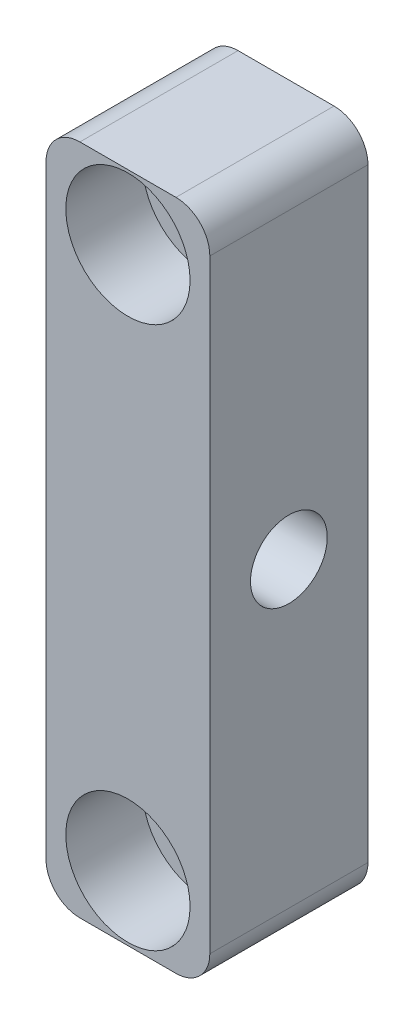
from build123d import *

# Parameters (mm, degrees)
SKETCH_1_W                = 14.5
SKETCH_1_H                = 59.5
EXTRUDE_1_DEPTH           = 14
FILLET_1_R                = 3
HOLE_WIZARD_2_D           = 6.6
HOLE_WIZARD_2_CBORE_D     = 11
HOLE_WIZARD_2_CBORE_DEPTH = 6.8
HOLE_WIZARD_M8_1_D        = 6.8


with BuildPart() as part:
    # 草图1 → 凸台-拉伸1 (new body)
    with BuildSketch(Plane.XY):
        Rectangle(SKETCH_1_W, SKETCH_1_H)
    extrude(amount=EXTRUDE_1_DEPTH)

    # 圆角1
    fillet_1_edges = [part.edges().sort_by_distance(p)[0] for p in [
        (7.25, -29.75, 7),
        (-7.25, -29.75, 7),
        (-7.25, 29.75, 7),
        (7.25, 29.75, 7),
    ]]
    fillet(fillet_1_edges, radius=FILLET_1_R)

    # 打孔尺寸(%根据)内六角圆柱头螺钉的类型2 (through all)
    with Locations(Plane.XY.offset(14)):
        with Locations((0, 24), (0, -24)):
            CounterBoreHole(HOLE_WIZARD_2_D / 2, HOLE_WIZARD_2_CBORE_D / 2, HOLE_WIZARD_2_CBORE_DEPTH)

    # M8 螺纹孔1 (through all)
    with Locations(Plane.ZY.offset(7.25)):
        with Locations((7, 0)):
            Hole(HOLE_WIZARD_M8_1_D / 2)


solid = part.part
